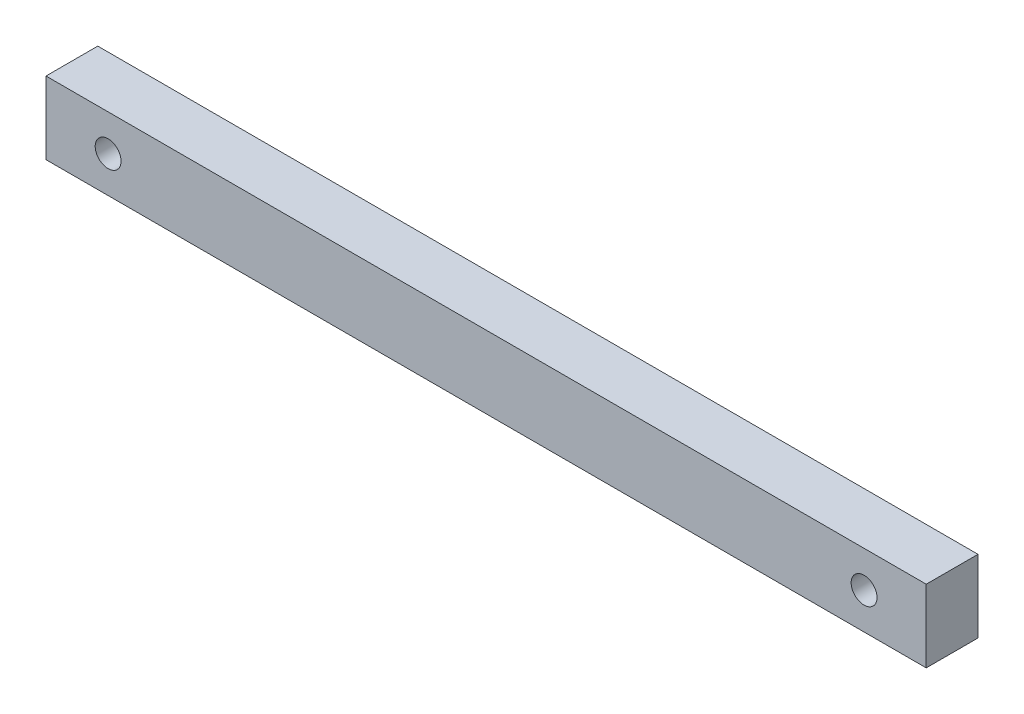
SolidWorks part; units mm, degrees
ref_plane "前视基准面" through (0, 0, 0) normal (0, 0, 1) x (1, 0, 0)
ref_plane "上视基准面" through (0, 0, 0) normal (0, 1, 0) x (1, 0, 0)
ref_plane "右视基准面" through (0, 0, 0) normal (1, 0, 0) x (0, 0, -1)
sketch "草图1" plane through (0, 0, 0) normal (0, 0, 1) x (1, 0, 0)
  line L1 (-85, -7) -> (85, -7)
  line L2 (-85, -7) -> (-85, 7)
  line L3 (-85, 7) -> (85, 7)
  line L4 (85, -7) -> (85, 7)
  line L5 (-85, -7) -> (85, 7) construction
  line L6 (-85, 7) -> (85, -7) construction
  point P0 (0, 0)
  dimension "D1" = 170
  dimension "D2" = 14
extrude "凸台-拉伸1" add sketch "草图1" along normal mid plane 10
hole_wizard "M6 螺纹孔1" positions "3D草图1" profile "草图2" tap size "M6" standard "GB" end condition up to next
sketch3d "3D草图1"
  line L0 (-85, 0, -5) -> (85, 0, -5) construction
  line L1 (-85, 7, -5) -> (-85, -7, -5) construction
  line L2 (85, -7, -5) -> (85, 7, -5) construction
  point P0 (-73, 0, -5)
  dimension "D1" = 12
sketch "草图2" plane through (-73, 0, -5) normal (1, 0, 0) x (0, 1, 0)
  line L0 (0, 0) -> (0, 10.001)
  line L1 (0, 10.001) -> (2.5, 10.001)
  line L2 (2.5, 10.001) -> (2.5, 0.525)
  line L3 (2.5, 0.525) -> (3.025, 0)
  line L5 (3.025, 0) -> (0, 0)
  line L6 (-2.5, 0.525) -> (-3.025, 0) construction
  line L11 (0, -6.35) -> (0, 107.95) construction
  dimension "通孔螺纹孔钻头直径" = 5
  dimension "通孔螺纹孔钻头深度" = 10.001
  dimension "近端锥形沉头孔直径" = 6.05
  dimension "近端锥形沉头孔角度" = 90
cosmetic thread "孔螺蚊线1" parameters "D2"=6
mirror "镜向1" about plane through (0, 0, 0) normal (1, 0, 0) of "M6 螺纹孔1"
